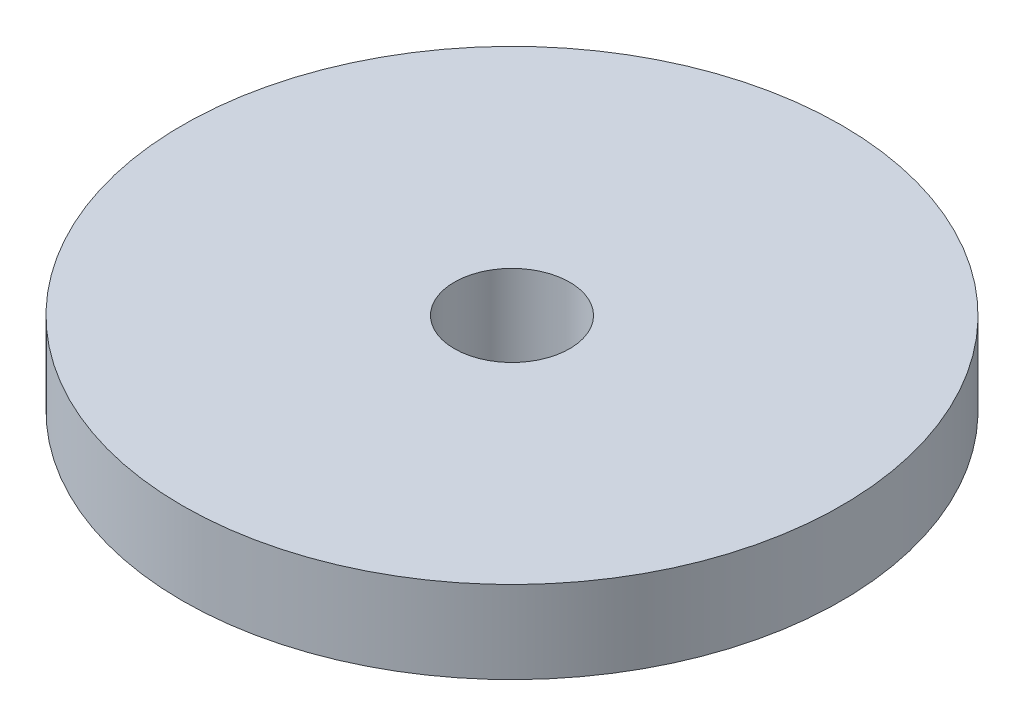
SolidWorks part; units mm, degrees
material "哈碳纤"
ref_plane "前视基准面" through (0, 0, 0) normal (0, 0, 1) x (1, 0, 0)
ref_plane "上视基准面" through (0, 0, 0) normal (0, 1, 0) x (1, 0, 0)
ref_plane "右视基准面" through (0, 0, 0) normal (1, 0, 0) x (0, 0, -1)
other "Configuration Table"
sketch "草图1" plane through (0, 0, 0) normal (0, 1, 0) x (1, 0, 0)
  circle A0 centre (0, 0) radius 12
  circle A1 centre (0, 0) radius 2.1
  dimension "D1" = 24
  dimension "D2" = 4.2
extrude "凸台-拉伸1" add sketch "草图1" along normal blind 3
